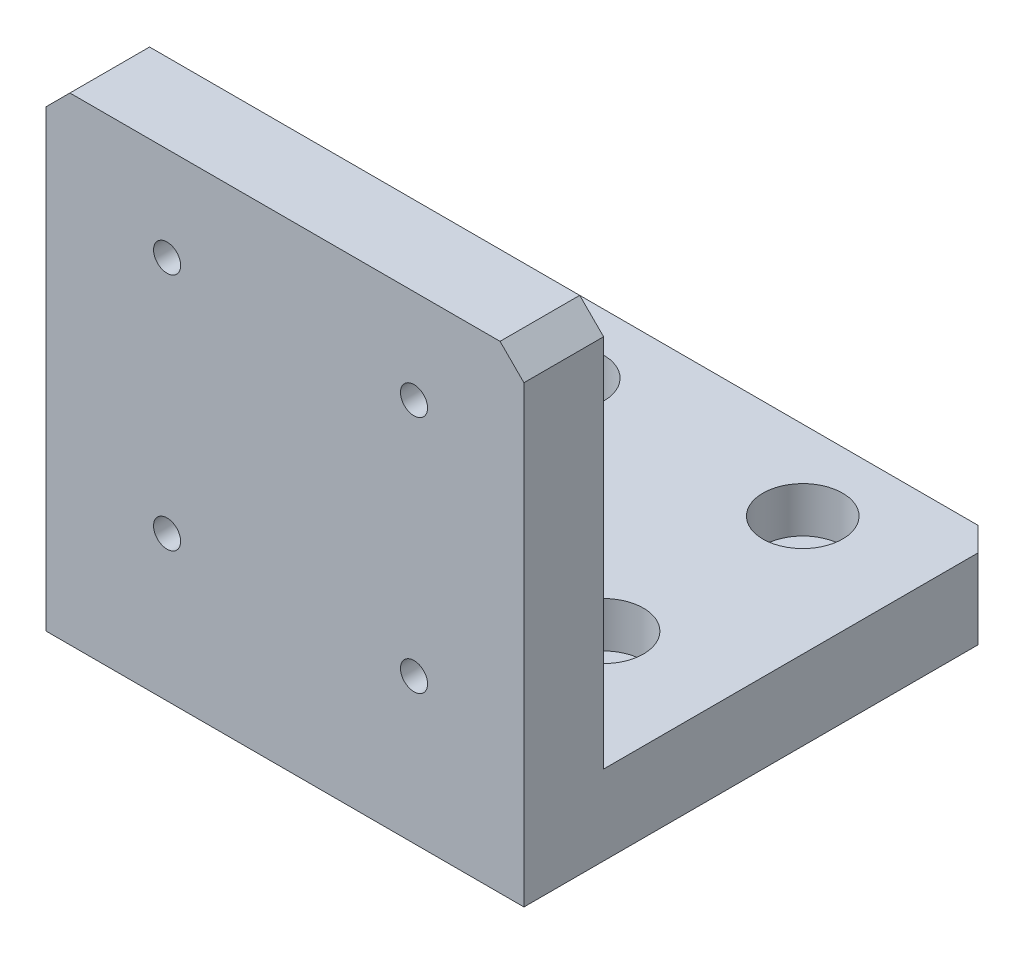
SolidWorks part; units mm, degrees
material "A6061 T6"
ref_plane "前视基准面" through (0, 0, 0) normal (0, 0, 1) x (1, 0, 0)
ref_plane "上视基准面" through (0, 0, 0) normal (0, 1, 0) x (1, 0, 0)
ref_plane "右视基准面" through (0, 0, 0) normal (1, 0, 0) x (0, 0, -1)
sketch "草图1" plane through (0, 0, 0) normal (0, 1, 0) x (1, 0, 0)
  line L1 (-30, 30) -> (30, 30)
  line L2 (-30, 30) -> (-30, -30)
  line L3 (-30, -30) -> (30, -30)
  line L4 (30, 30) -> (30, -30)
  line L5 (-30, 30) -> (30, -30) construction
  line L6 (-30, -30) -> (30, 30) construction
  point P0 (0, 0)
  dimension "D1" = 60
  dimension "D2" = 60
extrude "凸台-拉伸1" add sketch "草图1" along normal blind 10
sketch "草图2" plane through (0, 10, 0) normal (0, 1, 0) x (1, 0, 0)
  line L0 (30, -30) -> (30, 30) construction
  line L1 (-30, -30) -> (30, -30)
  line L2 (-30, -30) -> (-30, -20)
  line L3 (-30, -20) -> (30, -20)
  line L4 (30, -30) -> (30, -20)
  dimension "D1" = 10
extrude "凸台-拉伸2" add sketch "草图2" along normal blind 50
chamfer "倒角1" distance 3 angle 45 4 edges at (-30, 60, 25) (30, 60, 25) (30, 5, -30) (-30, 5, -30)
hole_wizard "打孔尺寸(%根据)内六角圆柱头螺钉的类型1" positions "草图3" profile "草图4" counterbore size "M5" standard "GB"
sketch "草图3" plane through (0, 10, 0) normal (0, 1, 0) x (1, 0, 0)
  line L0 (27, 30) -> (-27, 30) construction
  line L1 (-30, 27) -> (-30, -20) construction
  line L2 (30, -20) -> (30, 27) construction
  point P0 (-15, 20)
  point P2 (15, 20)
  point P4 (-15, -5)
  point P6 (15, -5)
  dimension "D1" = 10
  dimension "D2" = 15
  dimension "D3" = 15
  dimension "D4" = 25
sketch "草图4" plane through (-15, 10, -20) normal (1, 0, 0) x (0, 0, 1)
  line L0 (0, 0) -> (0, 16.6524)
  line L1 (0, 16.6524) -> (2.75, 15)
  line L2 (2.75, 15) -> (2.75, 5.7)
  line L3 (2.75, 5.7) -> (5, 5.7)
  line L4 (5, 5.7) -> (5, 0)
  line L5 (5, 0) -> (0, 0)
  line L10 (0, 16.6524) -> (-2.75, 15) construction
  line L11 (0, -6.35) -> (0, 107.95) construction
  dimension "孔直径" = 5.5
  dimension "孔深度" = 15
  dimension "柱形沉头孔直径" = 10
  dimension "柱形沉头孔深度" = 5.7
  dimension "导头角度" = 118
hole_wizard "打孔尺寸(%根据)内六角圆柱头螺钉的类型2" positions "草图5" profile "草图6" counterbore size "M3" standard "GB"
sketch "草图5" plane through (0, 0, 20) normal (0, 0, -1) x (-1, 0, 0)
  point P0 (-16.2, 48.2)
  point P3 (14.8, 48.2)
  point P6 (-16.2, 18.2)
  point P9 (14.8, 18.2)
sketch "草图6" plane through (16.2, 48.2, 20) normal (1, 0, 0) x (0, 1, 0)
  line L0 (0, 0) -> (0, 16.0215)
  line L1 (0, 16.0215) -> (1.7, 15)
  line L2 (1.7, 15) -> (1.7, 3.4)
  line L3 (1.7, 3.4) -> (3, 3.4)
  line L4 (3, 3.4) -> (3, 0)
  line L5 (3, 0) -> (0, 0)
  line L10 (0, 16.0215) -> (-1.7, 15) construction
  line L11 (0, -6.35) -> (0, 107.95) construction
  dimension "孔直径" = 3.4
  dimension "孔深度" = 15
  dimension "柱形沉头孔直径" = 6
  dimension "柱形沉头孔深度" = 3.4
  dimension "导头角度" = 118
